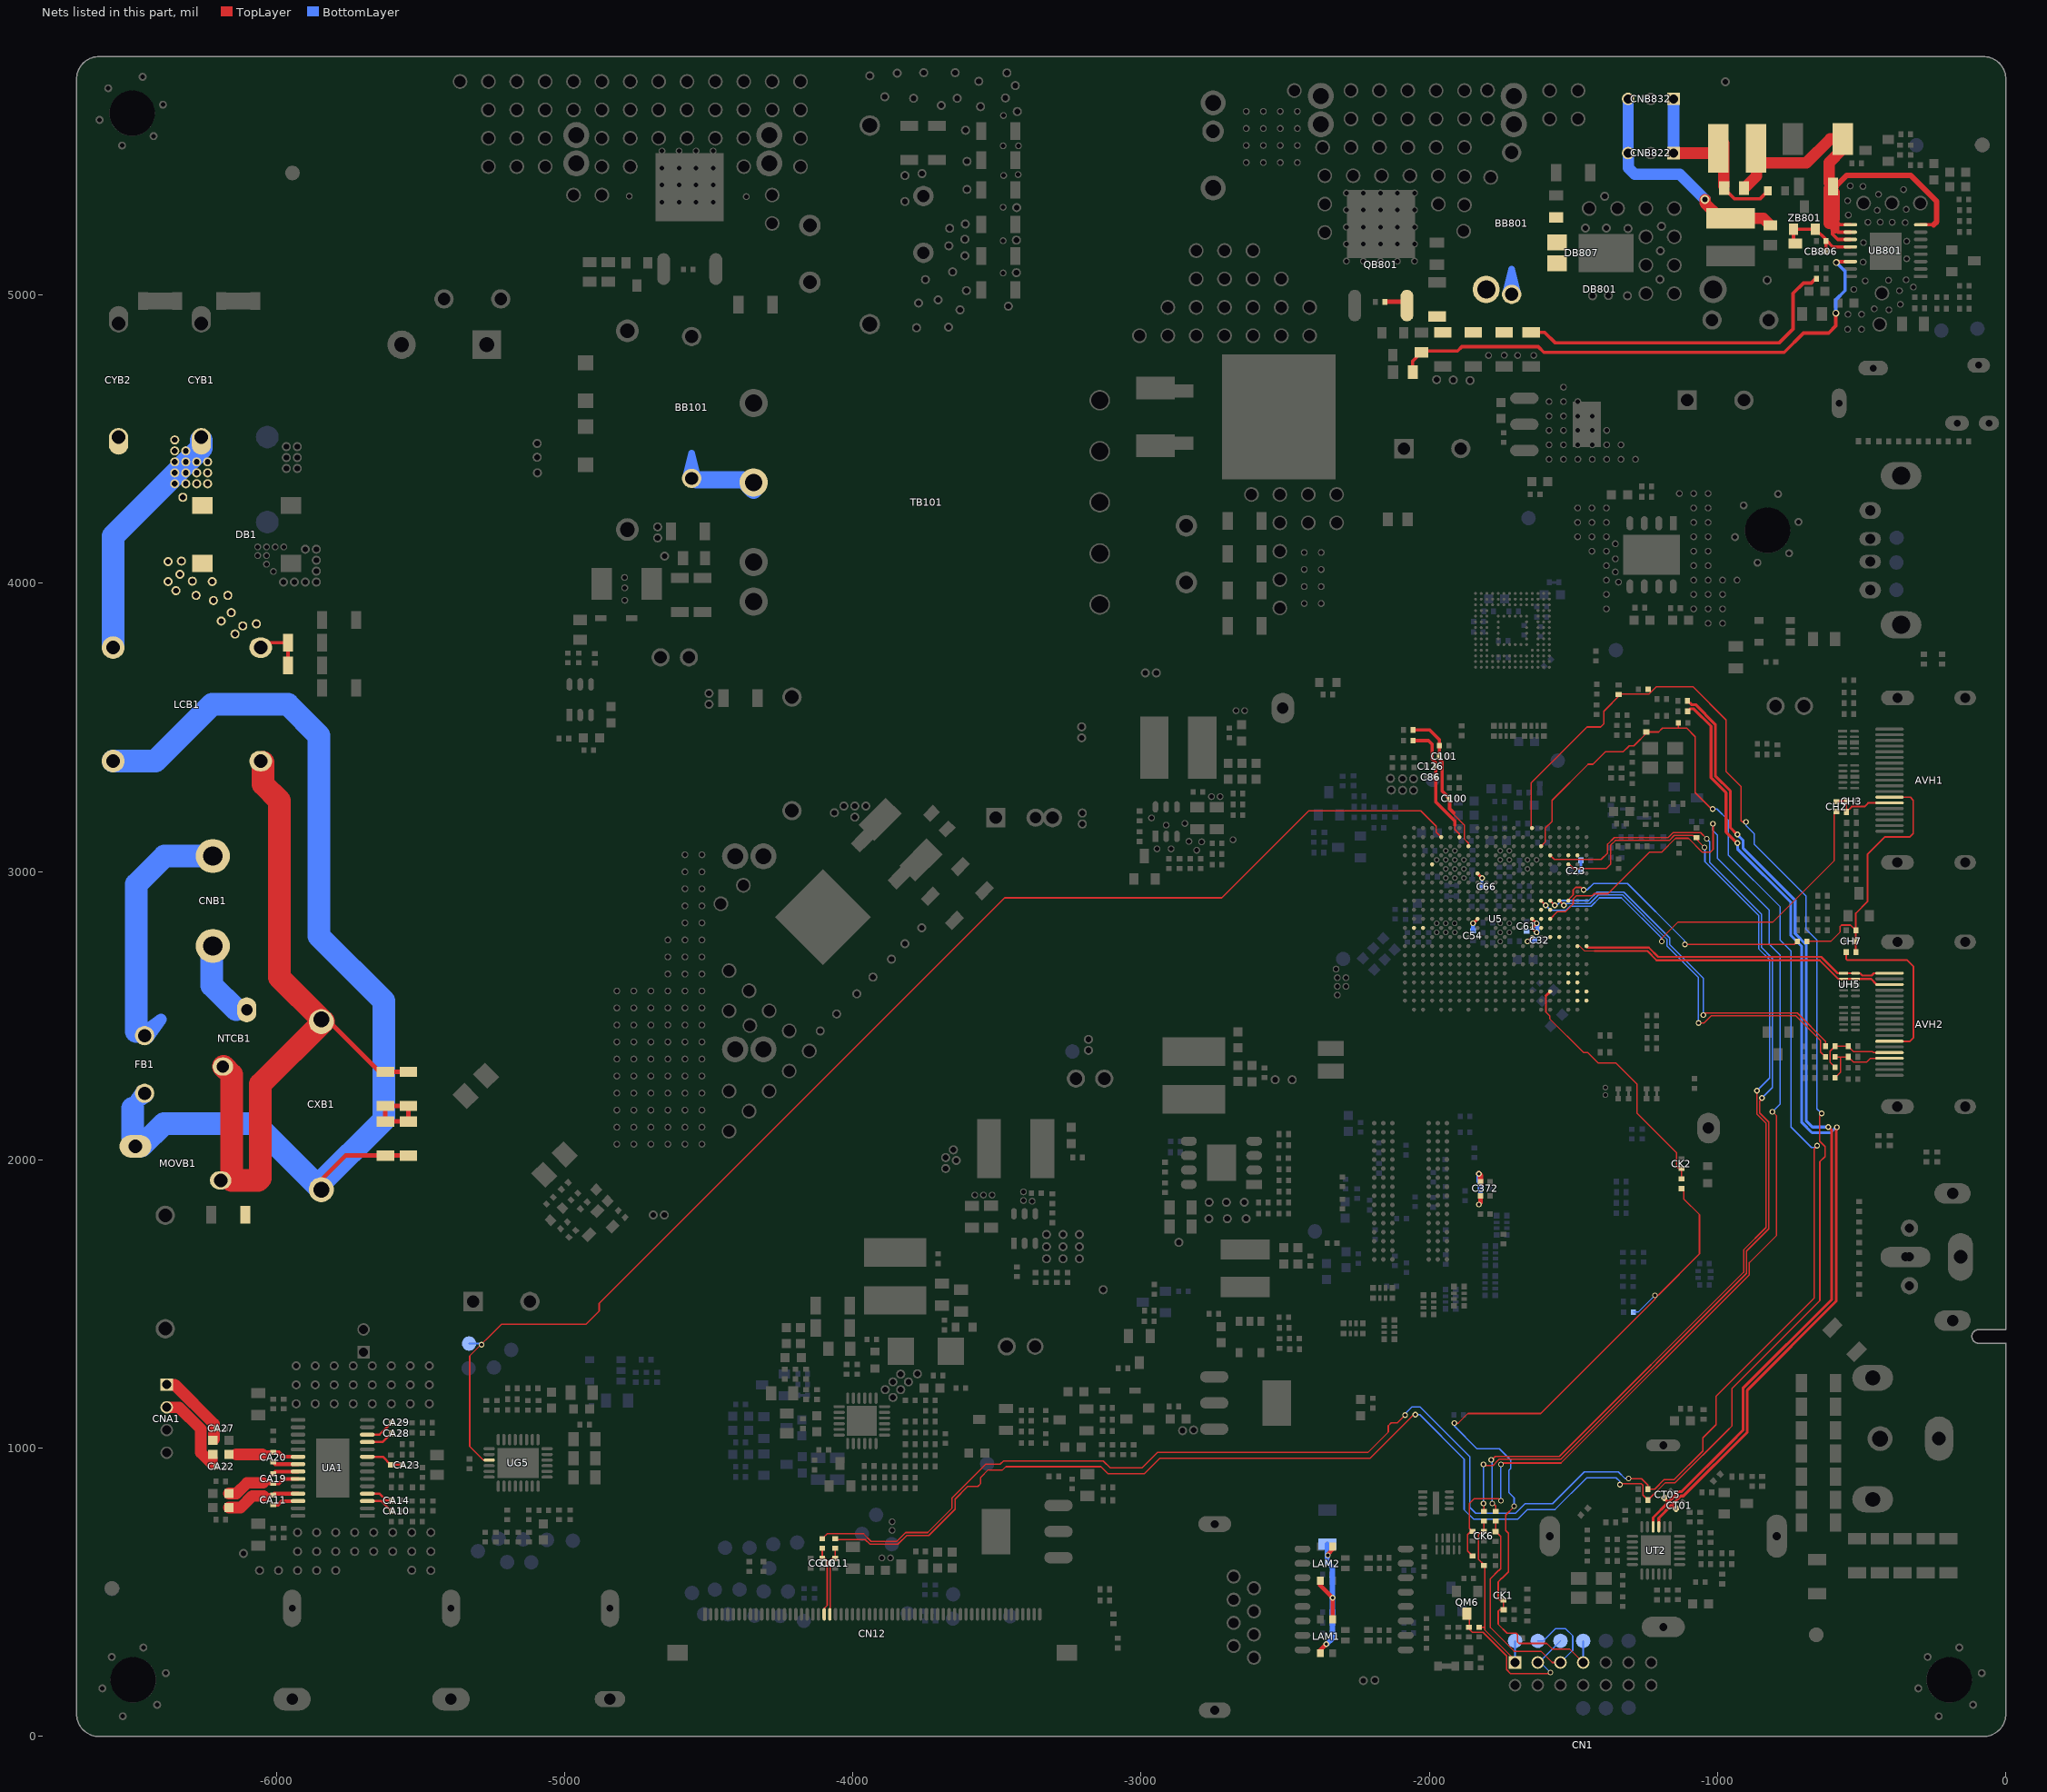
[diagram p0: the nets of this part, all layers, seen from the top]
# Altium PCB MISC84395.PcbDoc (part 20 of 26)
Units mil, origin at the board's own origin, x right, y up, seen from the top; angles counter-clockwise.
Board outline 6692.91 x 5826.77 mil, 2 copper layers (TopLayer, BottomLayer), stack 61.855 mil thick; 951 components, 565 nets, 4374 pads, 1804 vias.
Unrouted connection lines stored in the file: 1.

## Via types
v1: diameter 19.68, hole 11.81, TopLayer to BottomLayer, tented both sides, 1262 vias
v2: diameter 23.62, hole 15.75, TopLayer to BottomLayer, tented both sides, 524 vias
v3: diameter 31.5, hole 19.68, TopLayer to BottomLayer, tented both sides, 11 vias
v4: diameter 24, hole 16, TopLayer to BottomLayer, tented both sides, 6 vias
v5: diameter 19, hole 11.81, TopLayer to BottomLayer, tented both sides, 1 vias

## Nets (pads, with @x,y where several pads share a name; then routed paths per layer and width w, separated by ;. In a path a pad name is that pad's centre, name@x,y a point inside that pad or via, vN(x,y) a via of type N, cw(c..) or ccw(c..) an arc to the next point about the centre after c; other vN are vias at no path point) (continued)
HDMI2_RX2N_IC: AVH2.3 U5.H2 UH5.2 UH5.7 | length 1137.3
  TopLayer w3.94: -1478.63,2741.6 -1462.88,2725.85 -1427.21,2725.85
  TopLayer w4: U5.H2@-1486.5,2741.6 -1478.63,2741.6
  TopLayer w7: -1427.21,2724.34 -1243.62,2724.34 -1211.67,2692.4 -645.9,2692.4 -581.2,2627.7 UH5.2@-562.81,2627.7 UH5.7@-521.87,2627.7 -467.74,2627.7 -448.3,2608.27 AVH2.3@-403.84,2608.27
HDMI2_RX2P_IC: AVH2.1 U5.H1 UH5.1 UH5.8 | length 1096.7
  TopLayer w7: U5.H1@-1455.01,2741.6 -1449.76,2736.34 -1238.65,2736.34 -1206.7,2704.4 -640.93,2704.4 -583.92,2647.39 -506.24,2647.39 -498.56,2639.7 -465.87,2639.7 -457.93,2647.64 AVH2.1@-403.84,2647.64
HDMI2_SCL: AVH2.15 DH5.K RH14.2 RH17.1 | length 285.8
  TopLayer w5: -610.23,2338.59 -610,2338.35 ; RH14.2@-592.89,2321.24 -610,2338.35 ; AVH2.15@-403.84,2372.05 -458.81,2372.05 -462.68,2375.92 -529.03,2375.92 DH5.K@-547.36,2394.24 RH17.1@-592.89,2394.24 -610,2377.14 -610,2338.35
HDMI2_SCL_IC: RH17.2 U5.N5 | length 1307.3
  TopLayer w5: U5.N5@-1580.99,2899.08 v1(-1565,2883.09) v1@-1564.66,2882.74 ; v1(-1050,2502) -1042.6,2509.4 -1026.47,2509.4 -1003.82,2509.4 -723.67,2509.4 -626.36,2412.09 RH17.2@-626.36,2394.24
  BottomLayer w5: v1@-1564.65,2882.74 -1557.69,2882.74 -1541.03,2899.4 -1457,2899.4 -1447.61,2899.4 -1418.05,2928.96 -1325.49,2928.96 -1165.99,2769.46 -1165.99,2746.56 -1050.17,2630.73 v1@-1050.17,2502
HDMI2_SDA: AVH2.16 DH6.K RH15.2 RH16.1 | length 280.6
  TopLayer w5: RH15.2@-592.89,2285.24 -574.02,2304.11 -574.02,2355.84 ; RH16.1@-592.89,2357.24 DH6.K@-547.36,2357.24 -529.03,2338.92 -482.93,2338.92 -469.48,2352.36 AVH2.16@-403.84,2352.36
HDMI2_SDA_IC: RH16.2 U5.N4 | length 1329.6
  TopLayer w5: U5.N4@-1549.5,2899.08 v1(-1533.16,2882.74) ; v1(-1066,2475) -1047.59,2475 -1023.2,2499.4 -1022.33,2499.4 -1007.96,2499.4 -727.81,2499.4 -642.71,2414.31 -642.71,2373.6 RH16.2@-626.36,2357.24 RH16.2@-626.36,2354.9
  BottomLayer w5: v1(-1533.16,2882.74) -1526.5,2889.4 -1443.47,2889.4 -1413.91,2918.96 -1329.63,2918.96 -1176.3,2765.63 -1176.3,2742.73 -1067.51,2633.93 -1067.51,2476.51 v1(-1066,2475)
HDMI3_CLKN_IC: U5.B2
HDMI3_CLKP_IC: U5.B1
HDMI3_DET_IC: U5.M5
HDMI3_HPD_IC: U5.M6
HDMI3_RX0N_IC: U5.C1
HDMI3_RX0P_IC: U5.C2
HDMI3_RX1N_IC: U5.D3
HDMI3_RX1P_IC: U5.D2
HDMI3_RX2N_IC: U5.E3
HDMI3_RX2P_IC: U5.E2
HDMI3_SCL_IC: U5.L6
HDMI3_SDA_IC: U5.K6
HDMI_ARC: AVH1.14 CH2.1 CH3.2 DH1.K | length 243.5
  TopLayer w6: CH2.1@-585.27,3244.29 CH3.2@-553.38,3244.29 ; DH1.K@-553.38,3199.02 DH1.K@-553.38,3206.79 ; DH1.K@-553.38,3208.79 DH1.K@-553.38,3206.79 ; CH3.2@-553.38,3242.45 CH3.2@-553.38,3244.29 ; AVH1.14@-403.84,3238.19 -477.98,3238.19 -490.55,3225.62 -534.55,3225.62 DH1.K@-553.38,3206.79 ; DH1.K@-553.38,3206.79 CH3.2@-553.38,3244.29
HDMI_ARC_IC: CH2.2 U5.N6 | length 1414.2
  TopLayer w5: U5.N6@-1612.49,2899.08 v1(-1596.5,2883.09) ; v1(-1193.65,2757.74) -1193.65,2768.67 -1137.04,2825.28 -807.97,2825.28 -595.33,3037.92 -595.33,3200.76 CH2.2@-587.83,3208.26
  BottomLayer w5: v1(-1596.5,2883.09) -1578.81,2865.4 -1525.98,2865.4 -1511.98,2879.4 -1439.32,2879.4 -1409.76,2908.96 -1333.77,2908.96 -1195.65,2770.83 -1195.65,2759.74 v1(-1193.65,2757.74)
HDMI_CEC: AVH1.13 CH7.2 DH4.K RH9.2 RH13.1 | length 952.1
  TopLayer w5: RH13.1@-690.1,2758 -607.36,2758 -575.83,2789.53 -575.83,2808.49 -569.83,2814.49 -538.97,2814.49 DH4.K@-524.59,2800.11
  TopLayer w6: RH9.2@-520.54,2721 -520.63,2721.1 CH7.2@-520.63,2758.16 DH4.K@-520.64,2796.16 -520.64,2855.36 -479.38,2896.62 -479.38,3060.79 -420.39,3119.78 -334.37,3119.78 -321.53,3132.62 -321.53,3247.69 -331.71,3257.87 AVH1.13@-403.84,3257.87
HDMI_CEC2: AVH2.13 RH9.1 | length 604.1
  TopLayer w6: RH9.1@-554,2721 -554,2696 -550.47,2692.47 -342.63,2692.47 -320.53,2670.38 -320.53,2423.84 -332.95,2411.42 AVH2.13@-403.84,2411.42
HDMI_CEC_IC: RH13.2 U5.N3 | length 937
  TopLayer w5: U5.N3@-1518,2899.08 -1518,2902.35 -1501.09,2919.26 -1501.09,2936.61 -1492.54,2945.16 -1473.15,2945.16 v1(-1464.57,2936.58) ; v1@-1113.65,2747.4 -734.17,2747.4 RH13.2@-723.57,2758
  BottomLayer w5: v1@-1464.41,2936.74 -1452.69,2936.74 -1430.48,2958.96 -1313.06,2958.96 -1113.65,2759.54 v1(-1113.65,2747.74)
HP_OUTL_IC: U5.V2
HP_OUTR_IC: U5.V3
I2C_M_SCL_IC: D13.K RG18.1 RT10.1 RT39.1 U5.AA7 | length 7621.7
  TopLayer w5: RG18.1@-4061,686.73 -4057.52,683.25 -3956.72,683.25 -3940.47,667 -3843.3,667 -3812.8,697.5 -3736.24,697.5 -3645.5,788.24 -3645.5,823.73 -3601.73,867.5 -3566.52,867.5 -3556.36,877.66 -3556.36,898.72 -3530.48,924.61 -3480.55,924.61 -3469.16,936 -3139.28,936 -3115.28,912 -2988.19,912 -2935.19,965 -2205.26,965 v1@-2054,1116.26 ; U5.AA7@-1643.98,3151.04 -1647.18,3154.24 -1647.18,3171.45 -1647.47,3171.74 -1647.47,3307.06 -1453.13,3501.4 -1405.46,3501.4 -1394.71,3512.15 -1394.71,3556.15 -1335.35,3615.5 -1238.08,3615.5 -1213.24,3640.34 -1084.72,3640.34 -970.65,3526.27 -970.65,3347.13 -918.49,3294.98 -918.49,3176.32 -914.17,3172 v1(-901.83,3172) ; v1@-1336.68,876.32 -1263.77,876.32 -1259.38,871.93 -1259.38,837.1 RT10.1@-1242.27,820 -1181.58,880.68 -1146.98,880.68 -959.75,1067.91 ; -973.65,1054.02 -949.75,1077.91 -949.75,1207.96 -645.5,1512.22 -645.5,1993.97 -627.66,2011.82 -627.66,2046.04 -646.5,2064.88 -646.5,2153.49
  BottomLayer w5: v1(-2049,1116.26) -2033.26,1116.26 -1879.34,962.35 -1879.34,786.53 -1847.32,754.51 -1692.68,754.51 -1659.69,787.5 -1564.22,787.5 -1453.92,897.8 -1352.41,897.8 -1339,884.38 v1(-1339,874) ; v1(-901.83,3172) -901.83,3159.67 -873.81,3131.64 -873.81,3095.84 -693.96,2915.99 -693.96,2800.61 -655.5,2762.15 -655.5,2177.18 v1(-639.16,2160.84)
I2C_M_SDA_IC: D14.K RG19.1 RT5.1 RT40.1 U5.W6 | length 7500
  TopLayer w5: RG19.1@-4106,686.73 -4089.64,703.09 -3962.42,703.09 -3936.33,677 -3847.44,677 -3816.94,707.5 -3740.38,707.5 -3655.5,792.38 -3655.5,827.87 -3538.76,944.61 -3488.84,944.61 -3477.44,956 -3131,956 -3107,932 -2996.48,932 -2943.48,985 -2213.55,985 -2142.55,1055.99 -2142.55,1078.05 -2132.61,1088 -2111,1088 v1(-2084,1115) ; U5.W6@-1612.49,3088.05 -1597.9,3102.64 -1597.9,3150.49 -1574.65,3173.74 -1574.65,3246.83 -1449.23,3372.24 -1432.72,3372.24 -1389.56,3415.4 -1327.54,3415.4 -1306.69,3436.25 -1290.75,3436.25 -1243,3484 -1204.95,3484 -1191.49,3497.46 -1107.3,3497.46 -1077.65,3467.81 -1077.65,3273.97 v1@-1020.99,3217.32 ; v1(-1309,895) -1308,894 -1264,894 -1242.27,872.27 RT5.1@-1242.27,858 ; RT5.1@-1242.27,856.73 RT5.1@-1242.27,858 ; -1136.73,3498.56 RT40.1@-1136.73,3516 RT40.1@-1136.73,3519 ; v1(-655.16,2049.01) -665.5,2038.67 -665.5,1520.5 -1005.5,1180.5 -1005.5,1081.5 -1051.34,1035.66 -1051.34,990.46 -1151.12,890.68 -1185.73,890.68 -1218.41,858 RT5.1@-1242.27,858
  BottomLayer w5: v1(-2084,1115) -2084,1119.93 -2060.33,1143.61 -2032.32,1143.61 -1859.34,970.63 -1859.34,794.82 -1839.03,774.51 -1700.97,774.51 -1667.97,807.5 -1572.5,807.5 -1462.2,917.8 -1344.13,917.8 -1321.33,895 v1(-1309,895) ; v1@-1020.99,3217.32 v1(-1016.99,3217.32) -1002.44,3217.32 -963.49,3178.37 -963.49,3058.24 -783.96,2878.71 -783.96,2763.33 -745.5,2724.87 -745.5,2114.25 ; -745.5,2233.23 -745.5,2114.25 ; v1@-653.32,2043.33 -674.58,2043.33 -745.5,2114.25 ; v1@-651.4,2045.25 v1@-651.16,2045.01
I2C_SCL_PANEL: CG11.2 CN12.23 RG18.2 | length 243.6
  TopLayer w5: CN12.23@-4079.64,423.98 -4078.66,424.97 -4078.66,611.34 -4072.26,617.74 CG11.2@-4061,617.74 RG18.2@-4061,653.27
I2C_SDA_PANEL: CG10.2 CN12.22 RG19.2 | length 246.9
  TopLayer w5: RG19.2@-4106,653.27 CG10.2@-4106,617.73 -4095.73,617.73 -4088.66,610.66 -4088.66,455.34 -4099.33,444.67 CN12.22@-4099.33,423.98
I2S_OUT_SD_IC: U5.J4
I2S_OUT_WS_IC: U5.J5
IFN: CT05.2@-1180.96,832.04 CT05.2@-1185.83,827.16 RT2.1 UT2.10 | length 3399.9
  TopLayer w10: UT2.10@-1223.73,727.36 -1223.73,759.54 -1172.37,810.9 ; CT05.2@-1185.83,827.16 -1172.37,813.7 -1172.37,810.9 ; RT2.1@-1104.27,3592.13 -1091.14,3579 -1076.41,3579 -1008.15,3510.74 -1008.15,3331.6 -955.99,3279.44 -955.99,3152.16 v1@-932.94,3129.1 ; -959.64,1014.64 -955.54,1018.75 ; v1(-616,2114.13) -604,2102.13 -604,1516 -912.25,1207.75 -912.25,1062.04 -955.54,1018.75 ; -1172.37,810.9 -1143.04,840.24 -1134.06,849.22 -1125.07,849.22 -955.54,1018.75
  BottomLayer w10: v1@-931.15,3127.28 -911.31,3107.43 -911.31,3080.31 -731.46,2900.46 -731.46,2785.08 -693,2746.62 -693,2136 -671.13,2114.13 v1(-616,2114.13)
  other v1: -931.15,3129.1
IFP: CT01.2@-1139.96,794.04 CT01.2@-1144.83,789.16 RT4.1 UT2.9 | length 3435
  TopLayer w10: UT2.9@-1204.05,727.36 -1204.05,758.01 -1159.62,802.44 ; CT01.2@-1144.83,789.16 -1146.34,789.16 -1159.62,802.44 ; RT4.1@-1104,3556 -1096,3564 -1082.62,3564 -1023.15,3504.52 -1023.15,3325.39 -970.99,3273.23 -970.99,3137.16 -932.83,3099 -931.37,3099 v1(-931.15,3099.22) ; v1@-586,2105.34 v1(-586,2113.13) -589,2110.13 -589,1509.44 -897.25,1201.19 -897.25,1055.82 -1118.86,834.22 -1127.84,834.22 -1132.43,829.63 -1159.62,802.44
  BottomLayer w10: v1(-931.15,3099.22) -931.15,3078.93 -746.46,2894.24 -746.46,2778.87 -708,2740.41 -708,2129.79 -672.5,2094.29 -607.78,2094.29 -588.94,2113.13 v1(-586,2113.13)
IR: CK6.2 CN1.1 DK3.K IR.1 RK12.1 RK14.1 | length 649.9
  TopLayer w5: RK12.1@-1824,378.73 -1808.25,378.73 ; DK3.K@-1811,593.27 DK3.K@-1811,596.44 ; RK14.1@-1811,748.27 CK6.2@-1811,711.73 -1818.22,711.73 -1829.33,700.63 -1829.33,614.77 DK3.K@-1811,596.44 ; CN1.1@-1702.75,256.74 -1702.76,264.47 -1808.25,369.97 -1808.25,378.73 ; DK3.K@-1811,596.44 -1808.25,593.69 -1808.25,378.73
  BottomLayer w5: CN1.1@-1702.75,256.74 IR.1@-1702.7,332
IR_IN_IC: RK14.2 U5.V5 | length 3638.5
  TopLayer w5: v1(-1812.08,943.84) -1808.24,940 -1779.5,940 -1769.34,950.16 -1769.34,951.18 -1759.18,961.34 -1544.7,961.34 -1525.85,980.19 ; v1(-1812,808) -1811,809 RK14.2@-1811,780.73 ; U5.V5@-1578.67,3056.56 U5.V5@-1580.99,3056.56 -1566.4,3041.97 -1403.9,3041.97 -1381.65,3064.22 -1381.65,3094.92 -1358.73,3117.84 -1172.02,3117.84 -1154.52,3135.34 -1059.34,3135.34 v1(-1038,3114) ; -1525.91,980.24 -900,1606.15 -900,1683.78 -822.5,1761.28 -822.5,2131.29 -854,2162.79 -854,2203.51 -846,2211.51 v1(-846,2215)
  BottomLayer w5: v1(-1812.08,943.84) -1812,943.76 v1(-1812,808) ; v1(-1038,3114) -1027.49,3103.49 -1027.49,3031.74 -847.96,2852.2 -847.96,2736.82 -809.8,2698.67 -809.8,2251.2 v1(-846,2215)
KEY: CK1.1 CN1.7 DK1.K KEY.1 RK1.1 RK2.2 | length 2793.3
  TopLayer w5: v1(-1913,1087) -1899.92,1087 -1866.58,1120.34 -1613.5,1120.34 -1217.33,1516.51 v1(-1217.33,1530.32) ; -1761.25,389.95 -1761.25,389.44 ; DK1.K@-1743.34,436.62 -1743,436.96 DK1.K@-1743,439.62 ; CK1.1@-1743,477.27 CK1.1@-1743,473.27 ; v1(-1706,799) -1706,797.21 -1734.79,768.42 -1734.79,714.3 -1725.67,705.18 -1725.67,571.1 -1747.99,548.78 -1749.13,548.78 -1761.25,536.66 -1761.25,478 -1756.52,473.27 CK1.1@-1743,473.27 ; CN1.7@-1466.53,256.74 -1513.69,303.89 -1573.72,303.89 -1592.72,322.89 -1688.6,322.89 -1694.11,328.4 -1694.11,353.95 -1698.5,358.34 -1730.16,358.34 -1761.25,389.44 ; v1@-1212.14,1525.12 -1201.33,1535.94 -1063,1674.26 -1063,1810.25 -1118,1865.25 -1118,1893.27 RK2.2@-1124.99,1900.27 ; -1761.25,389.44 -1761.25,434.75 -1756.38,439.62 DK1.K@-1743,439.62 ; DK1.K@-1743,439.62 CK1.1@-1743,473.27
  BottomLayer w5: v1(-1913,1087) -1913,1076.62 -1834.88,998.5 -1757.41,998.5 -1717.66,958.75 -1717.66,929.77 -1724.34,923.09 -1724.34,846.2 -1706,827.86 v1(-1706,799) ; CN1.7@-1466.53,256.74 KEY.1@-1466.54,331.95 ; RK1.1@-1292.73,1472 -1275.65,1472 v1(-1217.33,1530.32)
KEY0_IN_IC: CK2.1 RK2.1 U5.C5 | length 931.5
  TopLayer w5: -1595.58,2569.53 -1595.58,2512.8 -1582.89,2500.11 -1582.89,2490.11 -1465.78,2373 -1451.43,2373 -1414.77,2336.34 -1353.17,2336.34 -1279.49,2262.67 -1279.49,2161.68 -1142.34,2024.53 -1142.34,1979 CK2.1@-1128.34,1965 ; -1142.34,1989 -1142.34,1975.83 -1138.51,1972 -1126.86,1972 CK2.1@-1125,1970.15 -1125,1937.15 RK2.1@-1123.29,1935.43
  TopLayer w10: -1595.58,2569.53 U5.C5@-1580.99,2584.12
L: CYB1.1 DB1.3 LCB1.2 pad.VIA5@-6238,4345 pad.VIA5@-6238,4383 pad.VIA5@-6238,4421 pad.VIA5@-6276,4345 pad.VIA5@-6276,4383 pad.VIA5@-6276,4421 pad.VIA5@-6314,4345 pad.VIA5@-6314,4383 pad.VIA5@-6314,4421 pad.VIA5@-6314,4459 pad.VIA5@-6324,4298 pad.VIA5@-6352,4345 pad.VIA5@-6352,4383 pad.VIA5@-6352,4421 pad.VIA5@-6352,4459 pad.VIA5@-6352,4497 | length 842.9
  BottomLayer w78.74: LCB1.2@-6565.91,3779.85 -6565.91,4163.09 -6260,4469 CYB1.1@-6260,4496
L-1: CNB1.1 FB1.1 | length 811.6
  BottomLayer w78.74: FB1.1@-6485,2446 -6485,2956 -6387.09,3053.91 CNB1.1@-6224,3053.91
L-2: CXB1.1 FB1.2 LCB1.3 MOVB1.1 RB1.1 RB2.1 | length 3831
  TopLayer w15.75: CXB1.1@-5878,1896.72 -5759.72,2015 RB1.1@-5565,2015
  BottomLayer w78.74: LCB1.3@-6565.81,3383 -6419,3383 -6222.15,3579.85 -5959.85,3579.85 -5852,3472 -5852,2776 -5627,2551 -5627,2138.72 -5856.32,1909.41 -6072.91,2126 -6389.69,2126 -6467.85,2047.85 -6498,2078 -6498,2180
L-N: RB1.2 RB2.2 RB3.1 RB4.1 | length 267.8
  TopLayer w15.75: RB2.2@-5621.63,2133.11 RB1.2@-5541.63,2133.11 RB3.1@-5541.63,2187 RB4.1@-5621.63,2187 RB2.2@-5621.63,2133.11
LC: LC.1 U5.Y17 UG5.11 | length 4664.6
  TopLayer w5: UG5.11@-5261.39,958.84 -5281.84,958.84 -5329,1006 -5329,1242 -5328.81,1242.19 -5328.81,1320.18 -5219.5,1429.5 -4926.43,1429.5 -4879.84,1476.09 -4879.84,1502.58 -3473.43,2909 -2720.43,2909 -2418.43,3211 -2029.77,3211 -1975.85,3157.09 -1975.85,3136.46 U5.Y17@-1958.94,3119.55
  BottomLayer w5: LC.1@-5331,1363 -5292,1363 v1(-5288,1359)
LCK_OUT_IC: U5.K19
LDE_OUT_IC: U5.K20
LED+: CNB822.3 CNB832.3 LB804.2 pad.VIA5@-1044,5331 RB824.2 | length 765.6
  TopLayer w39.37: pad.VIA5@-1044,5331 -1044,5319 LB804.2@-999,5274 ; LB804.2@-955,5264.96 -840.87,5264.96 RB824.2@-822.95,5247.05
  BottomLayer w39.37: CNB832.3@-1310.48,5679.74 CNB822.3@-1310.48,5492 -1310.22,5491.74 -1310.22,5441.22 -1287.74,5418.74 -1131.74,5418.74 pad.VIA5@-1044,5331
LED-: CNB822.1 CNB832.1 LB805.1 RB806.1 RB825.2 | length 702
  TopLayer w11.81: RB825.2@-977.09,5369 -941.09,5333 -853.78,5333 RB806.1@-825.78,5361
  TopLayer w40: CNB822.1@-1153,5492 -1012.96,5492 -979,5525.96 RB825.2@-979,5378
  BottomLayer w40: CNB832.1@-1153.26,5680 -1153,5679.74 CNB822.1@-1153,5492
LED_CS: QB801.S RB805.1 RB808.2 RB810.2 RB818.1 RB819.1 RB820.1 RB821.1 | length 1256.3
  TopLayer w11.81: RB820.1@-1632.49,4878.62 -1641,4870.11 -1600.11,4870.11 -1564.19,4834.19 -785.59,4834.19 -738.21,4881.56 -738.21,5005.52 -702.43,5041.3 -675.7,5041.3 -661,5056 RB805.1@-657.46,5056
  TopLayer w15.75: RB808.2@-2153.74,4976 -2090.74,4976 QB801.S@-2077.74,4963
LED_FB: DB802.A LB805.2 RB825.1 RB826.1 UB801.8 UB801.9 UB801.10 UB801.11 | length 1690.6
  TopLayer w11.81: -601.69,5228.87 -601.69,5210.5 -583.42,5192.24 UB801.11@-539.63,5192.24 ; -593.19,5228.87 -582.15,5217.83 UB801.10@-539.63,5217.83 ; -593.19,5260.87 -575.74,5243.42 UB801.9@-539.63,5243.42 ; UB801.8@-295.53,5243.42 -250.58,5243.42
  TopLayer w19.68: RB826.1@-595.94,5356 -595.94,5371.05 -552.15,5414.84 -330.85,5414.84 -240.16,5324.15 -240.16,5253.84 -250.58,5243.42
  TopLayer w31.5: -593.19,5228.87 -593.19,5260.87 -591.09,5262.96 RB826.1@-591.09,5356
  TopLayer w39.37: -613,5249 RB826.1@-613,5369
  TopLayer w40: RB825.1@-902.45,5375.45 -865.04,5412.87 LB805.2@-865.04,5478.04 ; LB805.2@-865.04,5508 LB805.2@-865.04,5478.04 ; RB826.1@-599.94,5376 -613,5389.06 -613,5459 -566.39,5505.61 DB802.A@-566.39,5541 -609.47,5541 -692.58,5457.88 -844.88,5457.88 LB805.2@-865.04,5478.04
LED_GATE: RB807.1 RB809.1 UB801.14 | length 1868.2
  TopLayer w11.81: RB809.1@-2057.81,4732 -2057.81,4771.09 RB807.1@-2028,4800.91 -2023.62,4805.28 -1902,4805.28 -1887,4820.28 -1622.28,4820.28 -1602.57,4800.57 -769.43,4800.57 -702,4868 -615,4868 -590,4893 v2(-590,4937) ; v2(-588,5112) -584.53,5115.47 UB801.14@-539.63,5115.47
  BottomLayer w11.81: v2(-590,4937) -590,4983 -558,5015 -558,5082 v2(-588,5112)
LED_OVP: CB806.2 RB803.2 RB814.1 UB801.12 ZB801.1 ZB801.3 | length 319.3
  TopLayer w11.81: RB814.1@-730,5178.09 -736.5,5184.59 ZB801.1@-736.5,5228 ZB801.3@-661.5,5228 -660.36,5228 -623.77,5191.42 RB803.2@-623.77,5190.52 ; CB806.2@-624.04,5150.89 RB803.2@-624.04,5190.25 ; RB803.2@-623.77,5186.52 RB803.2@-623.77,5189.99 ; UB801.12@-539.63,5166.65 -600.43,5166.65 RB803.2@-623.77,5189.99 ; RB803.2@-624.04,5190.25 RB803.2@-623.77,5190.52 ; RB803.2@-624.04,5190.25 RB803.2@-623.77,5189.99 ; RB803.2@-623.77,5189.99 RB803.2@-623.77,5190.52
LED_R: R37.2 RK8.1 U5.L5 | length 4205.5
  TopLayer w4: U5.L5@-1580.99,2836.08 U5.L5@-1580.99,2837.76
  TopLayer w5: RK8.1@-1850,626.73 -1867.34,644.07 -1867.34,700.66 -1856.27,711.73 R37.2@-1850,711.73 -1861,722.73 -1861,808.06 -1843.56,825.5 -1759.5,825.5 v1(-1752,818) ; v1@-1752,938 v1(-1752,944) ; v1@-1752,948.5 -1543.4,948.5 -890,1601.9 -890,1643.47 -795.5,1737.97 -795.5,2152.55 v1(-809.84,2166.89) ; U5.L5@-1577.9,2836.08 U5.L5@-1580.99,2836.08 -1556.4,2860.67 -1528.18,2860.67 -1501.09,2887.76 -1501.09,2905.12 -1490.22,2915.99 -1436.01,2915.99 -1429,2923 -1380.98,2923 -1237.11,3066.87 -1194.7,3066.87 -1146.23,3115.34 -1101.13,3115.34 -1052.66,3066.87 -1026.13,3066.87 -1015.83,3077.17 -1015.83,3168.05 v1@-1017.8,3170.02
  BottomLayer w5: v1(-1752,818) v1(-1752,944) ; v1@-1017.8,3170.02 -1016.24,3168.46 -1016.24,3142.5 -1000.49,3126.75 -1000.49,3045.75 -820.96,2866.21 -820.96,2748.01 -782.8,2709.85 -782.8,2193.93 ; v1(-809.84,2166.89) -782.8,2193.93 ; -782.8,2276 -782.8,2193.93
  other v1: -1016.83,3166.05
LED_R_M: CN1.3 LED_R.1 QM6.C RK5.2 | length 588.4
  TopLayer w5: RK5.2@-1868,378.73 -1850.89,361.63 -1814.05,361.63 -1731.91,279.48 -1731.91,231.98 ; RK5.2@-1861,378.73 QM6.C@-1861,417.47 ; -1727.52,227.59 -1731.91,231.98 ; v1(-1580,222.01) -1584.43,217.59 -1717.52,217.59 -1731.91,231.98
  BottomLayer w5: CN1.3@-1624.01,256.74 -1620.48,256.74 LED_R.1@-1545.28,331.94 ; CN1.3@-1614.73,256.74 v1(-1580,222.01)
LED_R_OFF: R34.2 RK4.1 U5.U3 | length 3546.8
  TopLayer w5: v1@-1786.68,955.71 -1771.05,971.34 -1548.95,971.34 -910,1610.3 -910,1687.92 -832.5,1765.42 -832.5,2127.15 -864,2158.65 v1(-864,2240) ; v1(-1782,808) -1778,808 -1770,800 RK4.1@-1770,780.73 ; U5.U3@-1518,3025.06 -1513.68,3025.06 -1499.09,3010.47 -1385.91,3010.47 -1371.65,3024.74 -1371.65,3090.78 -1354.59,3107.84 -1167.87,3107.84 -1150.38,3125.34 -1086.6,3125.34 v1(-1045.48,3084.22)
  BottomLayer w5: v1@-1786.68,955.71 -1782,951.03 v1(-1782,808) ; v1@-1050.48,3084.22 -1044.22,3077.95 -1044.22,3034.32 -857.96,2848.06 -857.96,2732.68 -819.8,2694.53 -819.8,2284.2 v1(-864,2240)
  other v1: -1785.68,959.71
LED_R_OFF_M: CN1.5 DU7.K LED_R_OFF.1 RK4.2 | length 945.8
  TopLayer w5: RK4.2@-1770,748.27 -1770,710.73 -1769.4,710.73 -1752.67,694 -1752.67,582.28 -1759.17,575.78 -1760.31,575.78 -1788.25,547.84 -1788.25,378.25 -1705.89,295.89 -1612.89,295.89 -1573.74,256.74 CN1.5@-1545.27,256.74
  BottomLayer w5: LED_R_OFF.1@-1624.02,331.94 -1605.38,331.94 -1562.88,374.44 -1527.67,374.44 -1502.78,349.55 -1502.78,299.24 CN1.5@-1545.27,256.74
LGND: CE5.1 LAM1.2 LAM1.4 LAM2.2 LAM2.4 RE1.1 RE2.1 RE3.1 RE4.1 | length 589.5
  TopLayer w15: LAM1.4@-2378.65,288.94 -2378.65,300.35 v1(-2358,321) ; LAM2.4@-2378.65,540.94 -2378.65,524.65 v1(-2335.35,481.35) LAM1.2@-2335.35,407.06 ; v1@-2352,633 -2335.35,649.65 LAM2.2@-2335.35,659.06
  BottomLayer w18: v1(-2358,321) -2355,321 -2336.27,339.73 RE2.1@-2336.27,358 RE3.1@-2336.27,432 -2336.27,587.27 -2354.05,605.05 CE5.1@-2354.05,666.94
  other v1: -2352,629
LOUT+: CA27.1 CNA1.1 LBA4.2 | length 283.6
  TopLayer w12: LBA4.2@-6215.92,1030.97 LBA4.2@-6208.81,1038.08
  TopLayer w40: CNA1.1@-6380,1220.47 -6352.47,1220.47 -6215.92,1083.92 LBA4.2@-6215.92,1030.97
LOUT-: CA22.2 CNA1.2 LBA3.2 | length 315
  TopLayer w12: CA22.2@-6208.75,937.06 LBA3.2@-6208.75,967.98
  TopLayer w40: CNA1.2@-6380,1141.73 -6337.37,1141.73 -6262,1066.36 -6262,985.11 -6224.1,947.21
LPO_WIFI_IC: U5.U18
N: CYB2.1 DB1.2 LCB1.1 pad.VIA5@-6069,3859 pad.VIA5@-6116,3852 pad.VIA5@-6143,3824 pad.VIA5@-6156,3898 pad.VIA5@-6168,3958 pad.VIA5@-6191,3869 pad.VIA5@-6218,3940 pad.VIA5@-6222,4006 pad.VIA5@-6278,3958 pad.VIA5@-6291,4007 pad.VIA5@-6329,4077 pad.VIA5@-6334,4031 pad.VIA5@-6348,3974 pad.VIA5@-6375,4006 pad.VIA5@-6375,4075 RB101.1 RB141.2 | length 181
  TopLayer w11.81: LCB1.1@-6054,3776.7 -6036.7,3794 RB141.2@-5959.32,3794 -5959.32,3715.38 RB101.1@-5958.94,3715
N-1: CNB1.3 NTCB1.2@-6102.29,2520.43 | length 256.3
  BottomLayer w78.74: CNB1.3@-6224,2742.09 -6224,2605.53 -6139.32,2520.85
N-2: CXB1.2 LCB1.4@-6054,3383 MOVB1.2@-6193,1929 NTCB1.1 RB3.2 RB4.2 RB5.2 | length 2472.5
  TopLayer w15.75: CXB1.2@-5836.68,2480.32 -5816.32,2480.32 -5641.11,2305.11 RB4.2@-5621.63,2305.11 RB3.2@-5565,2305.11
  TopLayer w78.74: NTCB1.1@-6182.63,2324 -6153.99,2295.36 -6153.99,1929 -6062.63,1929 -6054.63,1937 -6054.63,2262.37 -5836.68,2480.32 CXB1.2@-5843.63,2487.28 -5989,2632.65 -5989,3246.06 -6046.47,3303.53 LCB1.4@-6046.47,3378.53
NetBB101_2: BB101.2 TB101.3@-4344.32,4349.41 | length 213.8
  BottomLayer w59.06: BB101.2@-4542.74,4359 -4381.46,4359 TB101.3@-4344.32,4321.85
NetBB801_2: BB801.2 CB810.2 DB801.A DB807.1 DB807.3
NetC23_2: C23.2 R26.2 | length 35.5
  BottomLayer w8: C23.2@-1474.38,3003.28 R26.2@-1474.38,3038.74
NetC32_2: C32.2 U5.J7 | length 51.5
  TopLayer w10: v1(-1659.73,2757.34) U5.J7@-1643.98,2773.09
  BottomLayer w10: v1(-1659.73,2757.34) -1636.11,2757.34 -1633.17,2760.28 C32.2@-1632.17,2761.28
NetC54_1: C54.1 U5.L13 | length 48.2
  TopLayer w10: v1(-1848.71,2820.34) U5.L13@-1832.96,2836.08
  BottomLayer w15: C54.1@-1848.71,2794.53 C54.1@-1848.65,2794.47 -1848.65,2820.27 v1(-1848.71,2820.34)
NetC61_2: C61.2 pad.VIA5@-1628.24,2788.84 pad.VIA5@-1628.24,2820.34 U5.K7 U5.L7 | length 98.3
  TopLayer w10: U5.L7@-1643.98,2836.08 pad.VIA5@-1628.24,2820.34 U5.K7@-1643.98,2804.59 pad.VIA5@-1628.24,2788.84
  BottomLayer w5: pad.VIA5@-1628.24,2820.08 pad.VIA5@-1628.24,2820.34
  BottomLayer w19.68: pad.VIA5@-1628.24,2788.84 pad.VIA5@-1628.24,2820.08
NetC66_1: C66.1 U5.T13 | length 57.8
  TopLayer w10: U5.T13@-1832.96,2993.56 v1(-1817.21,2977.82)
  BottomLayer w10: v1@-1820.48,2981.09 v1(-1817.21,2977.82) ; C66.1@-1817.38,2946.74 v1@-1817.38,2977.65
NetC86_1: C86.1 C126.1 R46.1 U5.Y15 | length 432.1
  TopLayer w5: -1911.7,3160.87 -1911.7,3146.16 -1895.95,3130.42 U5.Y15@-1895.95,3119.55
  TopLayer w12: R46.1@-2056.27,3454 -2003,3454 -1990.54,3441.54 -1990.54,3390.5 -1977.91,3377.87 -1977.91,3241.91 -1911.7,3175.7 -1911.7,3160.87
NetC100_2: C100.2 C101.1 R48.2 R49.1 U5.W14 | length 514.5
  TopLayer w5: -1917.65,3200.74 -1879.04,3162.13 -1879.04,3113.51 -1864.46,3098.92 U5.W14@-1864.46,3088.05
  TopLayer w12: R48.2@-2056.27,3491 -1999,3491 -1965.38,3457.38 R49.1@-1965.38,3436.74 -1965.38,3389.38 -1955.8,3379.8 -1955.8,3278.8 C100.2@-1930,3253 -1930,3218.04 -1915.17,3203.21
NetC372_2: C372.2 MR300.1 MR301.1 | length 173.2
  TopLayer w15: v1(-1827.76,1845.51) -1822.8,1850.47 MR300.1@-1822.8,1875.45
  TopLayer w19.69: v1(-1828.37,1951.84) -1822.8,1946.28 MR301.1@-1822.8,1923.58
  BottomLayer w15: v1(-1827.76,1845.51) -1822.8,1850.47 C372.2@-1822.81,1901.09
  BottomLayer w17: v1(-1828.37,1951.84) -1828.37,1926.29 -1822.8,1920.72 C372.2@-1822.81,1901.09
NetCA10_1: CA10.1 UA1.3 | length 97.9
  TopLayer w8: UA1.3@-5684.07,816.78 -5635.42,816.78 CA10.1@-5600.6,781.96
NetCA11_1: CA11.1 LBA1.1 UA1.25 | length 260
  TopLayer w13: -6044.23,834.62 -6041.19,837.67 CA11.1@-6010.59,837.67 -6005.89,842.37 UA1.25@-5924.23,842.37
  TopLayer w40: LBA1.1@-6164.21,794.06 -6123.47,794.06 -6082.91,834.62 -6044.23,834.62
NetCA11_2: CA11.2 UA1.26 | length 91.6
  TopLayer w13: CA11.2@-6010.59,804.2 -5994.03,804.2 -5981.45,816.78 UA1.26@-5924.23,816.78
NetCA14_1: CA14.1 UA1.4 | length 93.2
  TopLayer w8: UA1.4@-5684.07,842.37 -5642.61,842.37 -5619.19,818.96 CA14.1@-5600.6,818.96
NetCA19_1: CA19.1 LBA2.1 UA1.23 | length 270
  TopLayer w13: -6054.28,878.21 CA19.1@-6010.6,878.21 -5990.99,878.21 -5975.64,893.55 UA1.23@-5924.23,893.55
  TopLayer w40: LBA2.1@-6164.21,843.06 -6138.11,843.06 -6101.55,879.62 -6045.8,879.62
NetCA19_2: CA19.2 UA1.22 | length 89.5
  TopLayer w13: CA19.2@-6010.6,911.68 -6003.13,919.15 UA1.22@-5924.23,919.15
NetCA20_1: CA20.1 LBA3.1 UA1.20 | length 214.1
  TopLayer w13: -6041.34,985.67 CA20.1@-6010.59,985.67 -5990.87,985.67 -5975.53,970.33 UA1.20@-5924.23,970.33
  TopLayer w40: -6138.85,978.78 -6048.23,978.78
NetCA20_2: CA20.2 UA1.21 | length 89.5
  TopLayer w13: CA20.2@-6010.59,952.2 -6003.13,944.74 UA1.21@-5924.23,944.74
NetCA23_1: CA23.1 RA11.1 UA1.9 | length 138.6
  TopLayer w8: UA1.9@-5684.07,970.33 -5630.46,970.33 RA11.1@-5602.61,942.48 CA23.1@-5556.97,942.48
NetCA28_1: CA28.1 UA1.11 | length 96.1
  TopLayer w8: UA1.11@-5684.07,1021.51 -5631.03,1021.51 CA28.1@-5600.6,1051.95
NetCA29_1: CA29.1 UA1.12 | length 100.8
  TopLayer w8: UA1.12@-5684.07,1047.1 -5642.44,1047.1 CA29.1@-5600.6,1088.94